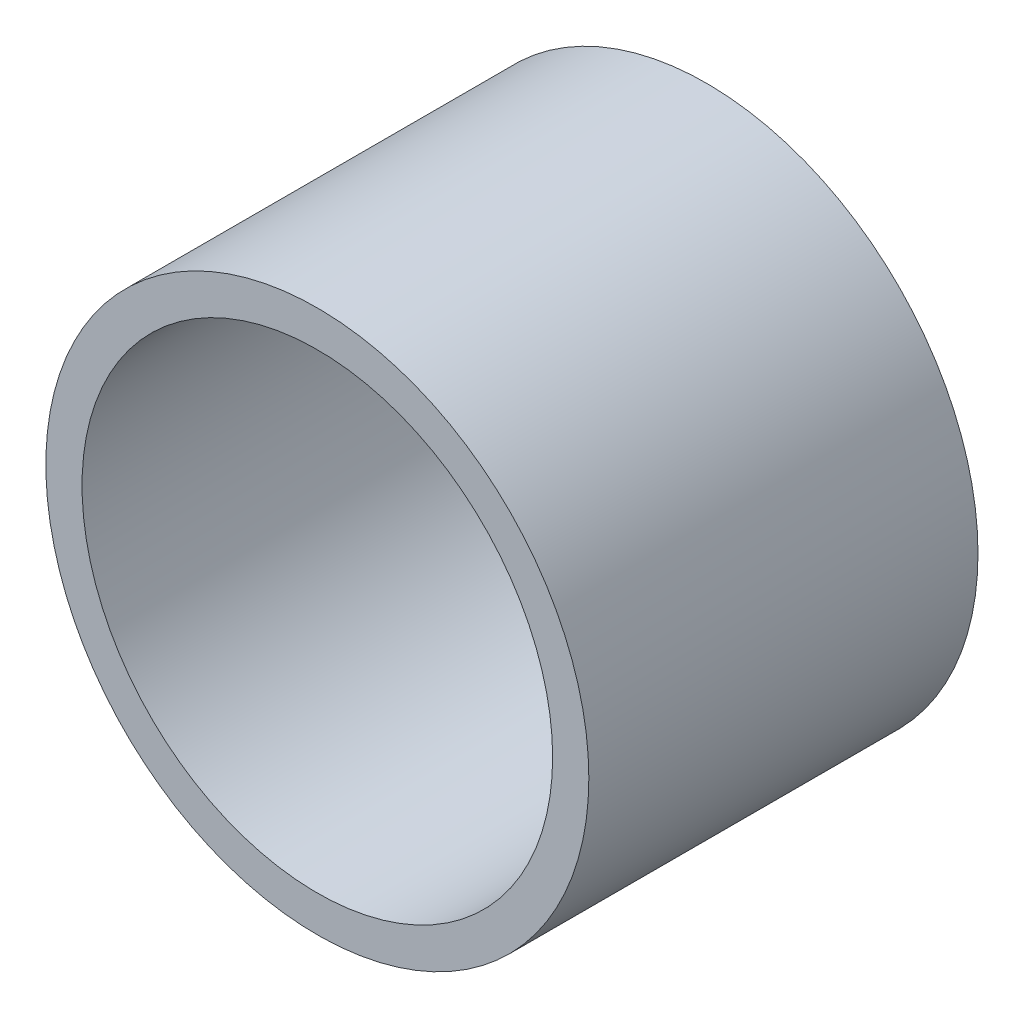
from build123d import *

# Parameters (mm, degrees)
SKETCH1_R           = 15
SKETCH1_R_2         = 13
BOSS_EXTRUDE1_DEPTH = 21.5


with BuildPart() as part:
    # Sketch1 → Boss-Extrude1 (new body)
    with BuildSketch(Plane.XY):
        Circle(SKETCH1_R)
        Circle(SKETCH1_R_2, mode=Mode.SUBTRACT)
    extrude(amount=BOSS_EXTRUDE1_DEPTH)


solid = part.part
